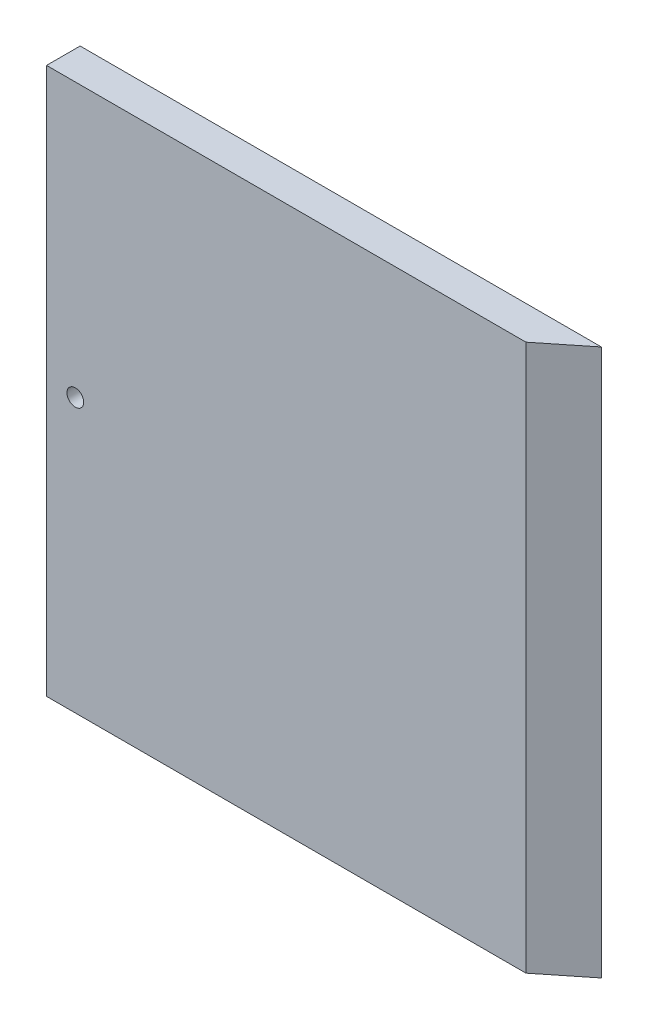
from build123d import *

# Parameters (mm, degrees)
SKETCH1_W           = 1000
SKETCH1_H           = 570
BOSS_EXTRUDE1_DEPTH = 35
M20_TAPPED_HOLE1_D  = 17.5
CUT_EXTRUDE2_DEPTH  = 1152.575008412


with BuildPart() as part:
    # Sketch1 → Boss-Extrude1 (new body)
    with BuildSketch(Plane.XY):
        with Locations((500, 285)):
            Rectangle(SKETCH1_W, SKETCH1_H)
    extrude(amount=BOSS_EXTRUDE1_DEPTH)

    # M20 Tapped Hole1 (through all)
    with Locations(Plane(origin=(30, 285, 35), x_dir=(1, 0, 0), z_dir=(0, 0, 1))):
        with Locations((0, 0)):
            Hole(M20_TAPPED_HOLE1_D / 2)

    # Sketch4 → Cut-Extrude2 (cut, through all)
    with BuildSketch(Plane.XZ):
        Polygon((500, 35), (1000, 35), (1000, -365), align=None)
    extrude(amount=-CUT_EXTRUDE2_DEPTH, mode=Mode.SUBTRACT)


solid = part.part
